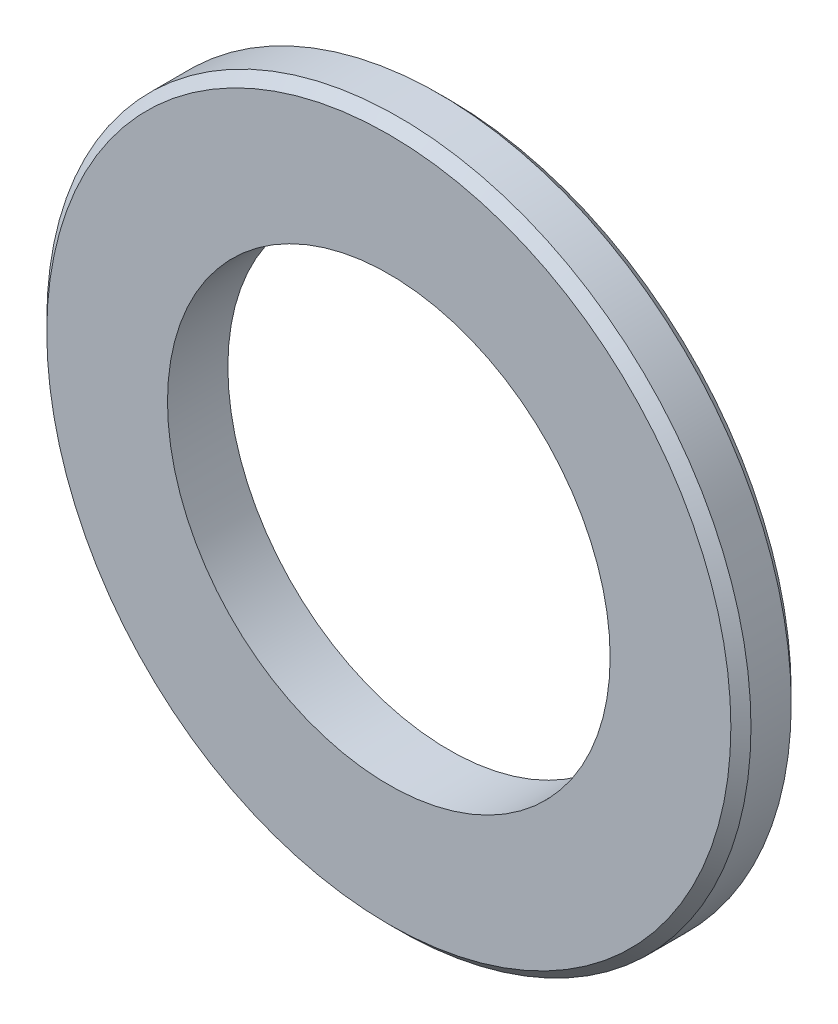
SolidWorks part; units mm, degrees
ref_plane "前视基准面" through (0, 0, 0) normal (0, 0, 1) x (1, 0, 0)
ref_plane "上视基准面" through (0, 0, 0) normal (0, 1, 0) x (1, 0, 0)
ref_plane "右视基准面" through (0, 0, 0) normal (1, 0, 0) x (0, 0, -1)
sketch "草图1" plane through (0, 0, 0) normal (0, 0, 1) x (1, 0, 0)
  circle A0 centre (0, 0) radius 17.5
  circle A1 centre (0, 0) radius 11
extrude "拉伸1" add sketch "草图1" along normal blind 3
chamfer "倒角1" distance 0.5 angle 45 2 edges at (17.5, 0, 0) (17.5, 0, 3)
